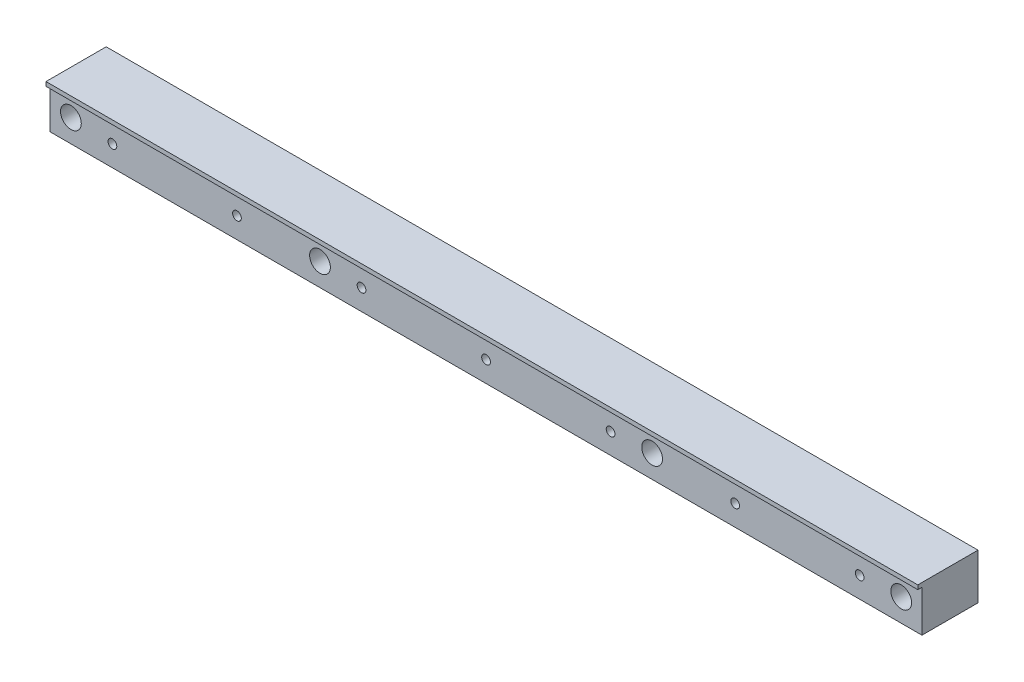
from build123d import *

# Parameters (mm, degrees)
SKETCH1_W                                           = 420
SKETCH1_H                                           = 22
BOSS_EXTRUDE1_DEPTH                                 = 27
SKETCH2_W                                           = 420
SKETCH2_H                                           = 2
BOSS_EXTRUDE2_DEPTH                                 = 2
M5_TAPPED_HOLE1_D                                   = 4.2
M5_TAPPED_HOLE1_DEPTH                               = 12.4
M5_TAPPED_HOLE1_TIP                                 = 1.2618073
CBORE_FOR_M5_HEX_SOCKET_HEAD_CAP_SCREW1_D           = 5.5
CBORE_FOR_M5_HEX_SOCKET_HEAD_CAP_SCREW1_CBORE_D     = 10
CBORE_FOR_M5_HEX_SOCKET_HEAD_CAP_SCREW1_CBORE_DEPTH = 17


with BuildPart() as part:
    # Sketch1 → Boss-Extrude1 (new body)
    with BuildSketch(Plane.XY):
        Rectangle(SKETCH1_W, SKETCH1_H)
    extrude(amount=BOSS_EXTRUDE1_DEPTH)

    # Sketch2 → Boss-Extrude2 (add)
    with BuildSketch(Plane.XY.offset(27)):
        with Locations((0, 10)):
            Rectangle(SKETCH2_W, SKETCH2_H)
    extrude(amount=BOSS_EXTRUDE2_DEPTH)

    # M5 Tapped Hole1
    with Locations(Plane.XY.offset(27)):
        with Locations((180, -1), (120, -1), (60, -1), (0, -1), (-180, -1), (-120, -1), (-60, -1)):
            Hole(M5_TAPPED_HOLE1_D / 2, depth=M5_TAPPED_HOLE1_DEPTH)
            with Locations((0, 0, -(M5_TAPPED_HOLE1_DEPTH + M5_TAPPED_HOLE1_TIP / 2))):  # 118° drill point
                Cone(0, M5_TAPPED_HOLE1_D / 2, M5_TAPPED_HOLE1_TIP, mode=Mode.SUBTRACT)

    # CBORE for M5 Hex Socket Head Cap Screw1 (through all)
    with Locations(Plane.XY.offset(27)):
        with Locations((200, 0), (80, 0), (-80, 0), (-200, 0)):
            CounterBoreHole(CBORE_FOR_M5_HEX_SOCKET_HEAD_CAP_SCREW1_D / 2, CBORE_FOR_M5_HEX_SOCKET_HEAD_CAP_SCREW1_CBORE_D / 2, CBORE_FOR_M5_HEX_SOCKET_HEAD_CAP_SCREW1_CBORE_DEPTH)


solid = part.part
